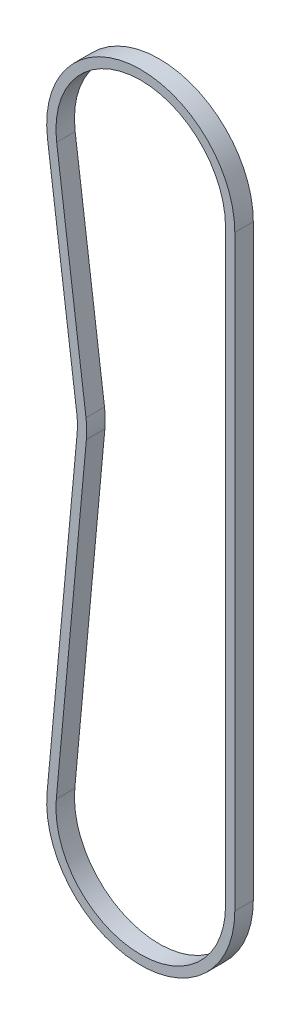
from build123d import *

# Parameters (mm, degrees)
EXTRUDE_1_DEPTH = 10


with BuildPart() as part:
    # 草图2 → 拉伸-薄壁1 (new, symmetric)
    with BuildSketch(Plane.XY):
        with BuildLine():
            Line((-69.067097429, -255.055208246), (-100.763322879, -13.205809086))
            ThreePointArc((-100.763322879, -13.205809085), (-6.616945736, 101.40935193), (101.624999966, 2.2e-08))
            Line((101.624999966, 2.2e-08), (101.624999966, -634.999999978))
            ThreePointArc((101.624999966, -634.999999978), (-4.66638799, -736.517808507), (-101.196460274, -625.677068041))
            Line((-101.196460274, -625.677068041), (-68.719202326, -273.150248716))
            ThreePointArc((-68.719202326, -273.150248716), (-68.390081735, -264.093056497), (-69.067097429, -255.055208246))
        make_face()
        with BuildLine():
            Line((-59.151887309, -253.755743635), (-90.848112759, -11.906344475))
            ThreePointArc((-90.848112759, -11.906344475), (-5.965831768, 91.430571914), (91.624999966, 2.2e-08))
            Line((91.624999966, 2.2e-08), (91.624999966, -634.999999978))
            ThreePointArc((91.624999966, -634.999999978), (-4.207210823, -726.528356253), (-91.238629008, -626.594453717))
            Line((-91.238629008, -626.594453717), (-58.76137106, -274.067634393))
            ThreePointArc((-58.76137106, -274.067634393), (-58.391929417, -263.900832101), (-59.151887309, -253.755743635))
        make_face(mode=Mode.SUBTRACT)
    extrude(amount=EXTRUDE_1_DEPTH, both=True)


solid = part.part
